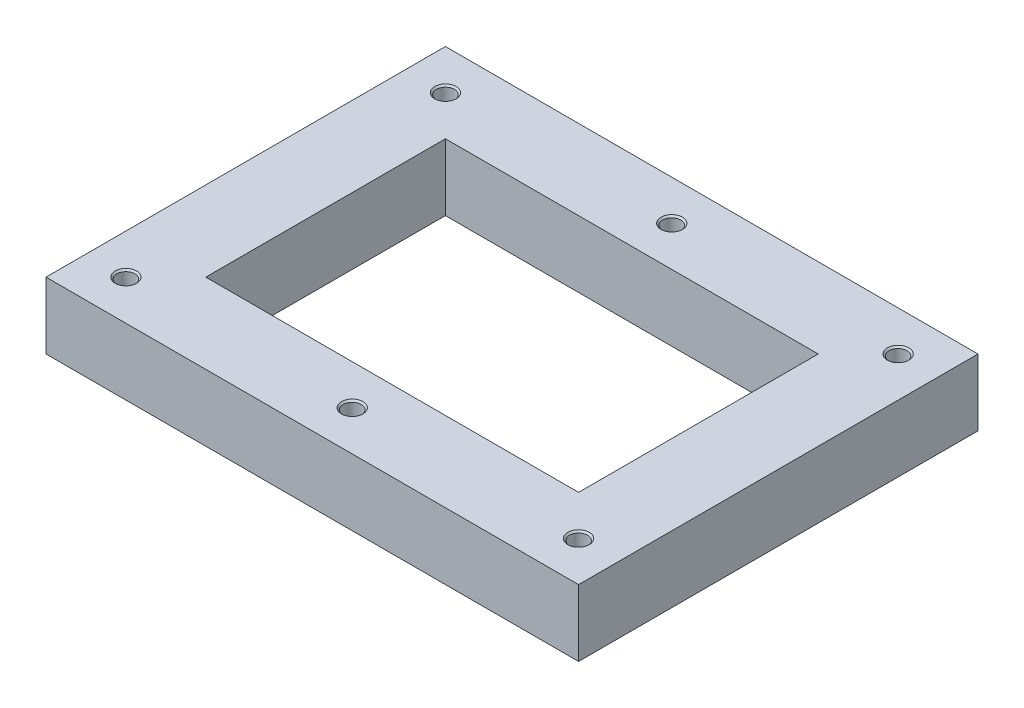
SolidWorks part; units mm, degrees
ref_plane "前视基准面" through (0, 0, 0) normal (0, 0, 1) x (1, 0, 0)
ref_plane "上视基准面" through (0, 0, 0) normal (0, 1, 0) x (1, 0, 0)
ref_plane "右视基准面" through (0, 0, 0) normal (1, 0, 0) x (0, 0, -1)
sketch "草图1" plane through (0, 0, 0) normal (0, 1, 0) x (1, 0, 0)
  line L1 (-100, 75) -> (100, 75)
  line L2 (-100, 75) -> (-100, -75)
  line L3 (-100, -75) -> (100, -75)
  line L4 (100, 75) -> (100, -75)
  line L5 (-100, 75) -> (100, -75) construction
  line L6 (-100, -75) -> (100, 75) construction
  point P0 (0, 0)
  dimension "D1" = 200
  dimension "D2" = 150
extrude "凸台-拉伸1" add sketch "草图1" along normal blind 25
hole_wizard "M8 螺纹孔1" positions "草图3" profile "草图4" tap size "M8" standard "GB"
sketch "草图3" plane through (0, 25, 0) normal (0, 1, 0) x (1, 0, 0)
  line L0 (-100, 75) -> (-100, -75) construction
  line L1 (0, 0) -> (100, 0) construction
  line L2 (100, -75) -> (100, 75) construction
  line L4 (-85, -60) -> (100, -60) construction
  point P0 (-85, -60)
  point P2 (0, -60)
  point P4 (85, -60)
  point P16 (85, 60)
  point P17 (0, 60)
  point P18 (-85, 60)
  point P23 (84.9902, -58.7105)
  dimension "D1" = 15
  dimension "D2" = 85
  dimension "D3" = 85
  dimension "D4" = 120
sketch "草图4" plane through (-85, 25, 60) normal (1, 0, 0) x (0, 0, 1)
  line L0 (0, 0) -> (0, 19.75)
  line L1 (0, 19.75) -> (3.4, 17.7071)
  line L2 (3.4, 17.7071) -> (3.4, 0.625)
  line L3 (3.4, 0.625) -> (4.025, 0)
  line L5 (4.025, 0) -> (0, 0)
  line L6 (-3.4, 0.625) -> (-4.025, 0) construction
  line L10 (0, 19.75) -> (-3.4, 17.7071) construction
  line L11 (0, -6.35) -> (0, 107.95) construction
  dimension "螺纹孔钻头直径" = 6.8
  dimension "螺纹孔钻头深度" = 19.75
  dimension "近端锥形沉头孔直径" = 8.05
  dimension "近端锥形沉头孔角度" = 90
  dimension "导头角度" = 118
cosmetic thread "孔螺蚊线1" parameters "D1"=16, "D2"=8
cosmetic thread "孔螺蚊线2" parameters "D1"=16, "D2"=8
cosmetic thread "孔螺蚊线3" parameters "D1"=16, "D2"=8
cosmetic thread "孔螺蚊线4" parameters "D1"=16, "D2"=8
cosmetic thread "孔螺蚊线5" parameters "D1"=16, "D2"=8
cosmetic thread "孔螺蚊线6" parameters "D1"=16, "D2"=8
sketch "草图5" plane through (0, 25, 0) normal (0, 1, 0) x (1, 0, 0)
  line L1 (70, 45) -> (-70, 45)
  line L2 (70, 45) -> (70, -45)
  line L3 (70, -45) -> (-70, -45)
  line L4 (-70, 45) -> (-70, -45)
  line L5 (70, 45) -> (-70, -45) construction
  line L6 (70, -45) -> (-70, 45) construction
  point P0 (0, 0)
  dimension "D1" = 140
  dimension "D2" = 90
extrude "切除-拉伸1" cut sketch "草图5" against normal through all both and the other way through all
